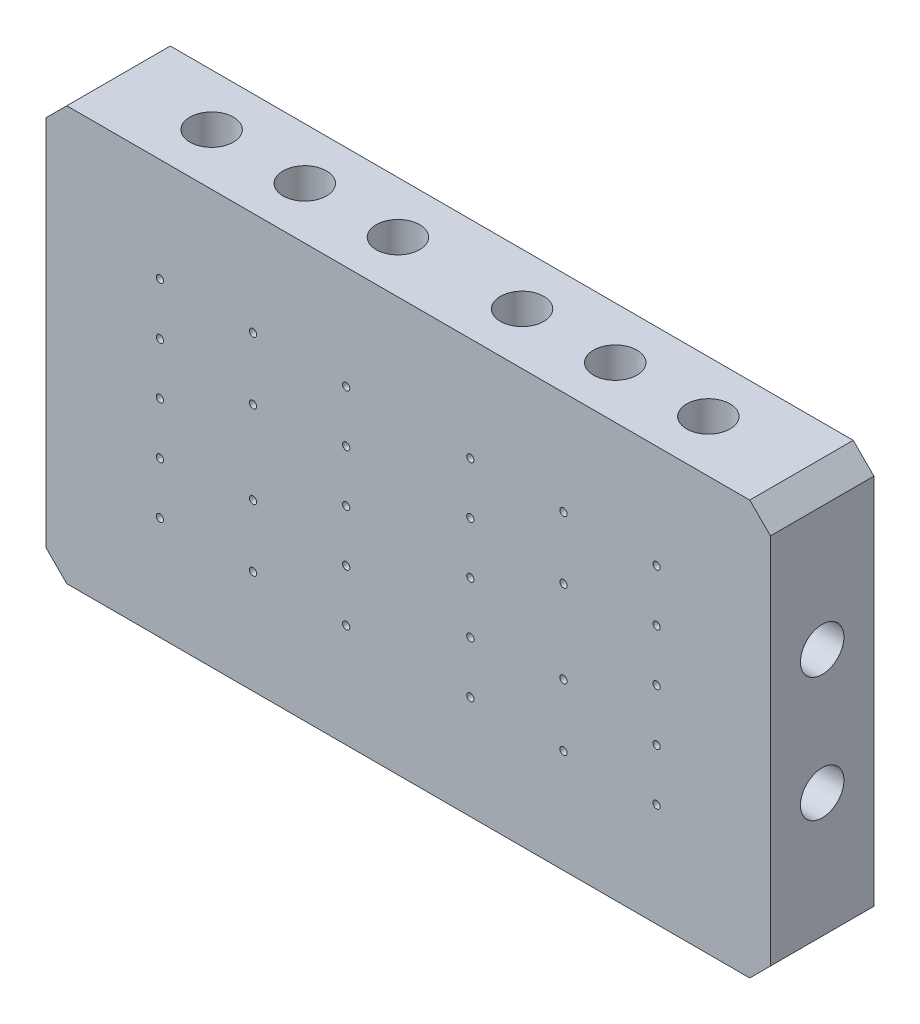
SolidWorks part; units mm, degrees
material "普通碳钢"
ref_plane "前基準面" through (0, 0, 0) normal (0, 0, 1) x (1, 0, 0)
ref_plane "上基準面" through (0, 0, 0) normal (0, 1, 0) x (1, 0, 0)
ref_plane "右基準面" through (0, 0, 0) normal (1, 0, 0) x (0, 0, -1)
sketch "草图1" plane through (0, 0, 0) normal (0, 0, 1) x (1, 0, 0)
  line L1 (-35, -20) -> (35, -20)
  line L2 (-35, -20) -> (-35, 20)
  line L3 (-35, 20) -> (35, 20)
  line L4 (35, -20) -> (35, 20)
  line L5 (-35, -20) -> (35, 20) construction
  line L6 (-35, 20) -> (35, -20) construction
  point P0 (0, 0)
  dimension "D1" = 70
  dimension "D2" = 40
extrude "凸台-拉伸1" add sketch "草图1" along normal blind 10
hole_wizard "Ø3.2 (3.2) 直径孔1" positions "草图2" profile "草图3" hole size "Ø3.2" standard "GB" end condition through all
sketch "草图2" plane through (35, 0, 0) normal (1, 0, 0) x (0, 0, -1)
  line L0 (0, 0) -> (-15.3599, 0) construction
  line L3 (-5, 20) -> (-5, -26.8477) construction
  line L4 (-10, 20) -> (0, 20) construction
  point P0 (-5, 6)
  point P2 (-5, -6)
  dimension "D1" = 12
sketch "草图3" plane through (35, 6, 5) normal (0, 1, 0) x (0, 0, -1)
  line L0 (0, 0) -> (0, 70)
  line L1 (0, 70) -> (1.6, 70)
  line L2 (1.6, 70) -> (1.6, 0)
  line L5 (1.6, 0) -> (0, 0)
  line L11 (0, -6.35) -> (0, 107.95) construction
  dimension "通孔孔直径" = 3.2
  dimension "通孔孔深度" = 70
hole_wizard "M5 螺纹孔1" positions "草图4" profile "草图5" tap size "M5" standard "GB"
sketch "草图4" plane through (35, 0, 0) normal (1, 0, 0) x (0, 0, -1)
  point P0 (-5, -6)
  point P3 (-5, 6)
sketch "草图5" plane through (35, -6, 5) normal (0, 1, 0) x (0, 0, -1)
  line L0 (0, 0) -> (0, 12.2618)
  line L1 (0, 12.2618) -> (2.1, 11)
  line L2 (2.1, 11) -> (2.1, 0)
  line L5 (2.1, 0) -> (0, 0)
  line L10 (0, 12.2618) -> (-2.1, 11) construction
  line L11 (0, -6.35) -> (0, 107.95) construction
  dimension "螺纹孔钻头直径" = 4.2
  dimension "螺纹孔钻头深度" = 11
  dimension "导头角度" = 118
cosmetic thread "孔螺蚊线1" parameters "D1"=8, "D2"=5
cosmetic thread "孔螺蚊线2" parameters "D1"=8, "D2"=5
hole_wizard "M5 螺纹孔2" positions "草图6" profile "草图7" tap size "M5" standard "GB"
sketch "草图6" plane through (-35, 0, 0) normal (-1, 0, 0) x (0, 0, 1)
  point P0 (5, 6)
  point P3 (5, -6)
sketch "草图7" plane through (-35, 6, 5) normal (0, 1, 0) x (0, 0, 1)
  line L0 (0, 0) -> (0, 13.2618)
  line L1 (0, 13.2618) -> (2.1, 12)
  line L2 (2.1, 12) -> (2.1, 0)
  line L5 (2.1, 0) -> (0, 0)
  line L10 (0, 13.2618) -> (-2.1, 12) construction
  line L11 (0, -6.35) -> (0, 107.95) construction
  dimension "螺纹孔钻头直径" = 4.2
  dimension "螺纹孔钻头深度" = 12
  dimension "导头角度" = 118
cosmetic thread "孔螺蚊线3" parameters "D1"=8, "D2"=5
cosmetic thread "孔螺蚊线4" parameters "D1"=8, "D2"=5
hole_wizard "Ø3.2 (3.2) 直径孔2" positions "草图8" profile "草图9" hole size "Ø3.2" standard "GB"
sketch "草图8" plane through (0, 20, 0) normal (0, 1, 0) x (1, 0, 0)
  line L0 (0, 0) -> (0, -13.1676) construction
  line L3 (35, -5) -> (-41.8267, -5) construction
  line L4 (35, -10) -> (35, 0) construction
  point P0 (-24, -5)
  point P2 (-15, -5)
  point P4 (-6, -5)
  point P26 (6, -5)
  point P27 (15, -5)
  point P28 (24, -5)
  dimension "D1" = 9
  dimension "D2" = 24
  dimension "D3" = 9
sketch "草图9" plane through (-24, 20, 5) normal (1, 0, 0) x (0, 0, 1)
  line L0 (0, 0) -> (0, 46.9614)
  line L1 (0, 46.9614) -> (1.6, 46)
  line L2 (1.6, 46) -> (1.6, 0)
  line L5 (1.6, 0) -> (0, 0)
  line L10 (0, 46.9614) -> (-1.6, 46) construction
  line L11 (0, -6.35) -> (0, 107.95) construction
  dimension "孔直径" = 3.2
  dimension "孔深度" = 46
  dimension "导头角度" = 118
sketch "草图10" plane through (0, 0, 10) normal (0, 0, 1) x (1, 0, 0)
  line L1 (-47.5, -20) -> (47.5, -20) construction
  line L2 (-47.5, -20) -> (-47.5, 20) construction
  line L3 (-47.5, 20) -> (47.5, 20) construction
  line L4 (47.5, -20) -> (47.5, 20) construction
  line L5 (-47.5, -20) -> (47.5, 20) construction
  line L6 (-47.5, 20) -> (47.5, -20) construction
  point P0 (0, 0)
  dimension "D1" = 95
  dimension "D2" = 40
hole_wizard "Ø0.7 (0.7) 直径孔2" positions "草图11" profile "草图12" hole size "Ø0.7" standard "GB"
sketch "草图11" plane through (0, 0, 10) normal (0, 0, 1) x (1, 0, 0)
  line L0 (0, 0) -> (-52.6326, 0) construction
  line L1 (-47.5, 20) -> (47.5, -20) construction
  line L4 (0, 0) -> (0, 27.5724) construction
  line L5 (-24, 0) -> (-24, 26.4409) construction
  line L6 (6, 0) -> (6, 27.0842) construction
  point P57 (-24, 0)
  point P59 (-24, 5)
  point P61 (-24, 10)
  point P71 (-24, -10)
  point P72 (-24, -5)
  point P74 (6, 10)
  point P76 (6, 5)
  point P78 (6, 0)
  point P89 (6, -5)
  point P91 (6, -10)
  dimension "D1" = 24
  dimension "D2" = 5
  dimension "D3" = 5
  dimension "D4" = 6
sketch "草图12" plane through (6, -10, 10) normal (1, 0, 0) x (0, -1, 0)
  line L0 (0, 0) -> (0, 5.2103)
  line L1 (0, 5.2103) -> (0.35, 5)
  line L2 (0.35, 5) -> (0.35, 0)
  line L5 (0.35, 0) -> (0, 0)
  line L10 (0, 5.2103) -> (-0.35, 5) construction
  line L11 (0, -6.35) -> (0, 107.95) construction
  dimension "孔直径" = 0.7
  dimension "孔深度" = 5
  dimension "导头角度" = 118
hole_wizard "Ø0.7 (0.7) 直径孔3" positions "草图19" profile "草图20" hole size "Ø0.7" standard "GB"
sketch "草图19" plane through (0, 0, 10) normal (0, 0, 1) x (1, 0, 0)
  line L0 (0, 0) -> (-50.8877, 0) construction
  line L1 (-47.5, -20) -> (47.5, 20) construction
  line L4 (0, 0) -> (0, 27.3483) construction
  line L7 (-15, 0) -> (-15, 30.4171) construction
  point P0 (-15, 10)
  point P2 (-15, 4)
  point P29 (-15, -4)
  point P31 (-15, -10)
  dimension "D1" = 15
  dimension "D2" = 6
  dimension "D3" = 4
sketch "草图20" plane through (-15, 10, 10) normal (1, 0, 0) x (0, -1, 0)
  line L0 (0, 0) -> (0, 5.2103)
  line L1 (0, 5.2103) -> (0.35, 5)
  line L2 (0.35, 5) -> (0.35, 0)
  line L5 (0.35, 0) -> (0, 0)
  line L10 (0, 5.2103) -> (-0.35, 5) construction
  line L11 (0, -6.35) -> (0, 107.95) construction
  dimension "孔直径" = 0.7
  dimension "孔深度" = 5
  dimension "导头角度" = 118
pattern_linear "阵列(线性)3" count 2 spacing 18 along (1, 0, 0) of "Ø0.7 (0.7) 直径孔2"
pattern_linear "阵列(线性)4" count 2 spacing 30 along (1, 0, 0) of "Ø0.7 (0.7) 直径孔3"
hole_wizard "M3 螺纹孔2" positions "草图21" profile "草图22" tap size "M3" standard "GB"
sketch "草图21" plane through (0, 0, 0) normal (0, 0, -1) x (-1, 0, 0)
  line L0 (0, 0) -> (0, 27.7361) construction
  line L2 (0, 0) -> (-52.8397, 0) construction
  point P0 (-30, 15)
  point P2 (0, 15)
  point P4 (30, 15)
  point P6 (-30, -15)
  point P8 (0, -15)
  point P10 (30, -15)
  dimension "D1" = 15
  dimension "D2" = 30
sketch "草图22" plane through (30, 15, 0) normal (1, 0, 0) x (0, 1, 0)
  line L0 (0, 0) -> (0, 8.2511)
  line L1 (0, 8.2511) -> (1.25, 7.5)
  line L2 (1.25, 7.5) -> (1.25, 0)
  line L5 (1.25, 0) -> (0, 0)
  line L10 (0, 8.2511) -> (-1.25, 7.5) construction
  line L11 (0, -6.35) -> (0, 107.95) construction
  dimension "螺纹孔钻头直径" = 2.5
  dimension "螺纹孔钻头深度" = 7.5
  dimension "导头角度" = 118
cosmetic thread "孔螺蚊线12" parameters "D1"=5, "D2"=3
cosmetic thread "孔螺蚊线13" parameters "D1"=5, "D2"=3
cosmetic thread "孔螺蚊线14" parameters "D1"=5, "D2"=3
cosmetic thread "孔螺蚊线15" parameters "D1"=5, "D2"=3
cosmetic thread "孔螺蚊线16" parameters "D1"=5, "D2"=3
cosmetic thread "孔螺蚊线17" parameters "D1"=5, "D2"=3
chamfer "倒角1" distance 2 angle 45 4 edges at (-35, 20, 5) (-35, -20, 5) (35, -20, 5) (35, 20, 5)
hole_wizard "M5 螺纹孔4" positions "草图23" profile "草图24" tap size "M5" standard "GB"
sketch "草图23" plane through (0, 20, 0) normal (0, 1, 0) x (1, 0, 0)
  point P0 (-24, -5)
  point P3 (-15, -5)
  point P6 (-6, -5)
  point P9 (6, -5)
  point P12 (15, -5)
  point P15 (24, -5)
sketch "草图24" plane through (-24, 20, 5) normal (1, 0, 0) x (0, 0, 1)
  line L0 (0, 0) -> (0, 13.2618)
  line L1 (0, 13.2618) -> (2.1, 12)
  line L2 (2.1, 12) -> (2.1, 0)
  line L5 (2.1, 0) -> (0, 0)
  line L10 (0, 13.2618) -> (-2.1, 12) construction
  line L11 (0, -6.35) -> (0, 107.95) construction
  dimension "螺纹孔钻头直径" = 4.2
  dimension "螺纹孔钻头深度" = 12
  dimension "导头角度" = 118
cosmetic thread "孔螺蚊线18" parameters "D1"=8, "D2"=5
cosmetic thread "孔螺蚊线19" parameters "D1"=8, "D2"=5
cosmetic thread "孔螺蚊线20" parameters "D1"=8, "D2"=5
cosmetic thread "孔螺蚊线21" parameters "D1"=8, "D2"=5
cosmetic thread "孔螺蚊线22" parameters "D1"=8, "D2"=5
cosmetic thread "孔螺蚊线23" parameters "D1"=8, "D2"=5
